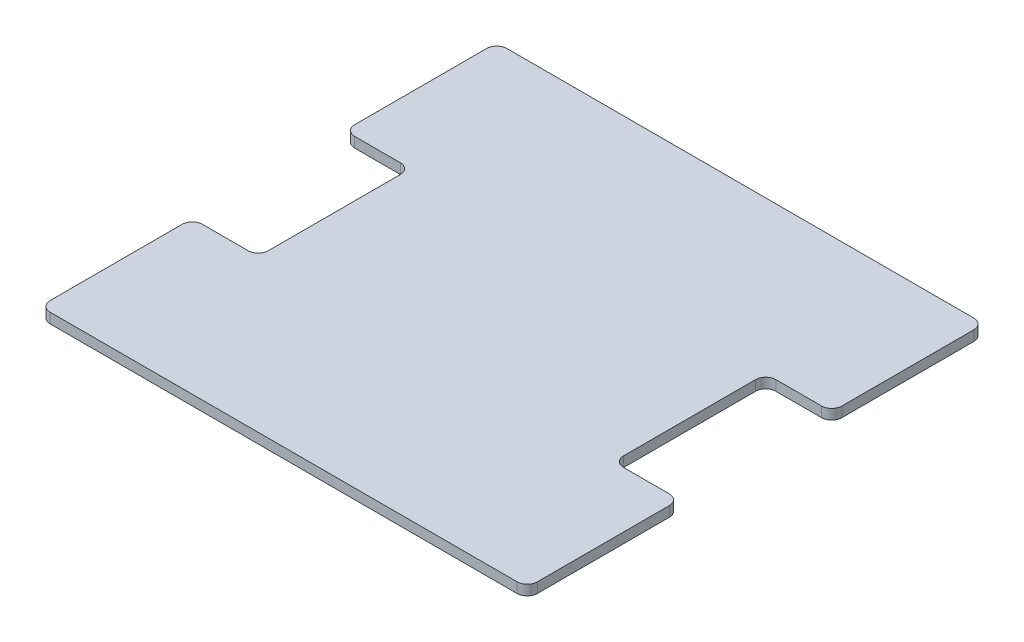
from build123d import *

# Parameters (mm, degrees)
SKETCH1_W           = 480
SKETCH1_H           = 650
BOSS_EXTRUDE1_DEPTH = 10
FILLET2_R           = 60
SKETCH3_W           = 130
SKETCH3_H           = 150
CUT_EXTRUDE1_DEPTH  = 10
SKETCH5_W           = 562.756234426
SKETCH5_H           = 100
CUT_EXTRUDE2_DEPTH  = 10
FILLET3_R           = 10


with BuildPart() as part:
    # Sketch1 → Boss-Extrude1 (new body)
    with BuildSketch(Plane(origin=(0, 0, 0), x_dir=(1, 0, 0), z_dir=(0, 1, 0))):
        Rectangle(SKETCH1_W, SKETCH1_H)
    extrude(amount=BOSS_EXTRUDE1_DEPTH)

    # Fillet2
    fillet2_edges = [part.edges().sort_by_distance(p)[0] for p in [
        (240, 5, 325),
        (-240, 5, 325),
        (-240, 5, -325),
        (240, 5, -325),
    ]]
    fillet(fillet2_edges, radius=FILLET2_R)

    # Sketch3 → Cut-Extrude1 (cut)
    with BuildSketch(Plane(origin=(0, 10, 0), x_dir=(1, 0, 0), z_dir=(0, 1, 0))):
        with Locations((240, 0)):
            Rectangle(SKETCH3_W, SKETCH3_H)
        with Locations((-240, 0)):
            Rectangle(SKETCH3_W, SKETCH3_H)
    extrude(amount=-CUT_EXTRUDE1_DEPTH, mode=Mode.SUBTRACT)

    # Sketch5 → Cut-Extrude2 (cut)
    with BuildSketch(Plane(origin=(0, 10, 0), x_dir=(1, 0, 0), z_dir=(0, 1, 0))):
        with Locations((0, -275)):
            Rectangle(SKETCH5_W, SKETCH5_H)
        with Locations((0, 275)):
            Rectangle(SKETCH5_W, SKETCH5_H)
    extrude(amount=-CUT_EXTRUDE2_DEPTH, mode=Mode.SUBTRACT)

    # Fillet3
    fillet3_edges = [part.edges().sort_by_distance(p)[0] for p in [
        (-240, 5, 75),
        (-175, 5, 75),
        (-240, 5, -75),
        (-175, 5, -75),
        (240, 5, -75),
        (175, 5, -75),
        (240, 5, 75),
        (175, 5, 75),
        (-240, 5, 225),
        (240, 5, -225),
        (240, 5, 225),
        (-240, 5, -225),
    ]]
    fillet(fillet3_edges, radius=FILLET3_R)


solid = part.part
